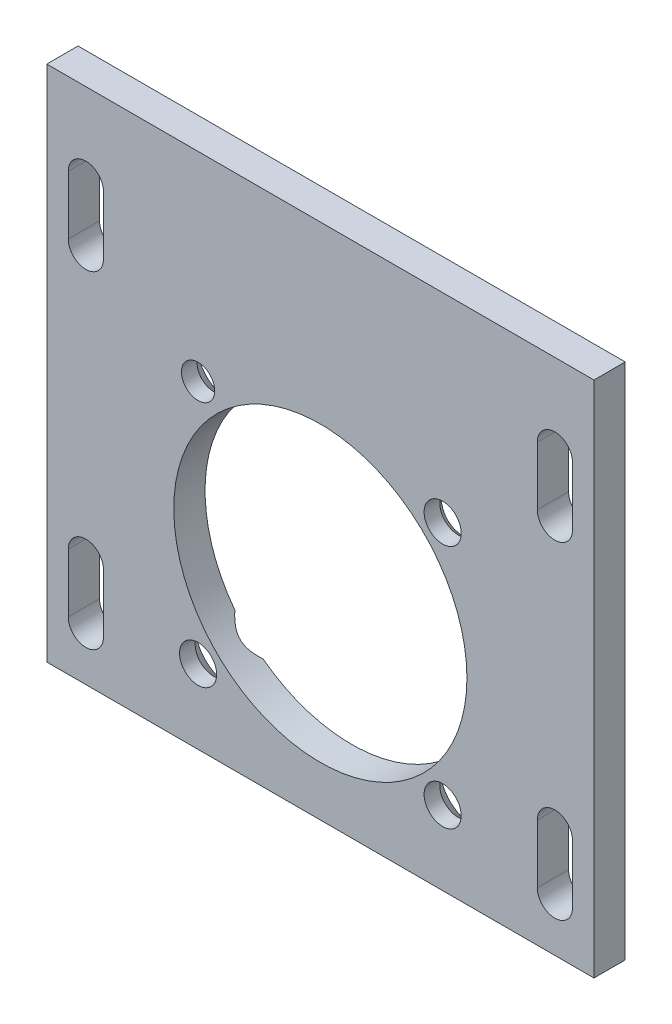
from build123d import *

# Parameters (mm, degrees)
SKETCH1_W                = 280
SKETCH1_H                = 280
SKETCH1_R                = 75
EXTRUDE1_DEPTH           = 8
SKETCH_2_2_R             = 8.5
SKETCH_2_2_R_2           = 9.5
EXTRUDE2_DEPTH           = 8
EXTRUDE4_START           = -8
SKETCH_2_2_2_R           = 8.5
EXTRUDE4_DEPTH           = 8
EXTRUDE4_DRAFT           = 45
SKETCH_2_2_2_R_2         = 9.5
EXTRUDE4_PROFILE_2_DEPTH = 8
EXTRUDE4_PROFILE_2_DRAFT = 45
EXTRUDE4_PROFILE_3_DEPTH = 8
EXTRUDE4_PROFILE_3_DRAFT = 45
EXTRUDE4_PROFILE_4_DEPTH = 8
EXTRUDE4_PROFILE_4_DRAFT = 45
SKETCH3_W                = 280
SKETCH3_H                = 15
EXTRUDE5_DEPTH           = 16


with BuildPart() as part:
    # Sketch1 → Extrude1 (new, symmetric)
    with BuildSketch(Plane.XY):
        with Locations((0, 24.5)):
            Rectangle(SKETCH1_W, SKETCH1_H)
        Circle(SKETCH1_R, mode=Mode.SUBTRACT)
        with BuildLine():
            Line((-129, 122.5), (-129, 92.5))
            ThreePointArc((-129, 92.5), (-120, 83.5), (-111, 92.5))
            Line((-111, 92.5), (-111, 122.5))
            ThreePointArc((-111, 122.5), (-120, 131.5), (-129, 122.5))
        make_face(mode=Mode.SUBTRACT)
        with BuildLine():
            Line((111, 122.5), (111, 92.5))
            ThreePointArc((111, 92.5), (120, 83.5), (129, 92.5))
            Line((129, 92.5), (129, 122.5))
            ThreePointArc((129, 122.5), (120, 131.5), (111, 122.5))
        make_face(mode=Mode.SUBTRACT)
        with BuildLine():
            Line((-129, -45), (-129, -75))
            ThreePointArc((-129, -75), (-120, -84), (-111, -75))
            Line((-111, -75), (-111, -45))
            ThreePointArc((-111, -45), (-120, -36), (-129, -45))
        make_face(mode=Mode.SUBTRACT)
        with BuildLine():
            Line((111, -45), (111, -75))
            ThreePointArc((111, -75), (120, -84), (129, -75))
            Line((129, -75), (129, -45))
            ThreePointArc((129, -45), (120, -36), (111, -45))
        make_face(mode=Mode.SUBTRACT)
    extrude(amount=EXTRUDE1_DEPTH, both=True)

    # Sketch 2_2 → Extrude2 (cut)
    with BuildSketch(Plane.XY.offset(8)):
        with Locations((-62.578950135, 62.578950135)):
            Circle(SKETCH_2_2_R)
        with Locations((62.578950135, 62.578950135)):
            Circle(SKETCH_2_2_R_2)
        with Locations((62.578950135, -62.578950135)):
            Circle(SKETCH_2_2_R_2)
        with Locations((-62.578950135, -62.578950135)):
            Circle(SKETCH_2_2_R_2)
    extrude(amount=-EXTRUDE2_DEPTH, mode=Mode.SUBTRACT)


with BuildPart() as extrude4_tool:
    # Sketch 2_2 2 → Extrude4 (with draft: the straight prism first)
    with BuildSketch(Plane.XY.offset(8).offset(EXTRUDE4_START)):
        with Locations((-62.578950135, 62.578950135)):
            Circle(SKETCH_2_2_2_R)
    extrude(amount=-EXTRUDE4_DEPTH)
    # Extrude4: the draft: its side faces are tilted about the plane it starts from
    extrude4_sides = [extrude4_tool.faces().sort_by_distance(p)[0] for p in [
        (-71.078950135, 62.578950135, -4),
    ]]
    draft(extrude4_sides, Plane.XY.offset(8).offset(EXTRUDE4_START), EXTRUDE4_DRAFT)


with BuildPart() as part_1:
    add(part.part)

    # Extrude4: cut by extrude4_tool
    add(extrude4_tool.part, mode=Mode.SUBTRACT)


with BuildPart() as extrude4_profile_2_tool:
    # Sketch 2_2 2 → Extrude4 profile 2 (with draft: the straight prism first)
    with BuildSketch(Plane.XY.offset(8).offset(EXTRUDE4_START)):
        with Locations((62.578950135, 62.578950135)):
            Circle(SKETCH_2_2_2_R_2)
    extrude(amount=-EXTRUDE4_PROFILE_2_DEPTH)
    # Extrude4 profile 2: the draft: its side faces are tilted about the plane it starts from
    extrude4_profile_2_sides = [extrude4_profile_2_tool.faces().sort_by_distance(p)[0] for p in [
        (53.078950135, 62.578950135, -4),
    ]]
    draft(extrude4_profile_2_sides, Plane.XY.offset(8).offset(EXTRUDE4_START), EXTRUDE4_PROFILE_2_DRAFT)


with BuildPart() as part_2:
    add(part_1.part)

    # Extrude4 profile 2: cut by extrude4_profile_2_tool
    add(extrude4_profile_2_tool.part, mode=Mode.SUBTRACT)


with BuildPart() as extrude4_profile_3_tool:
    # Sketch 2_2 2 → Extrude4 profile 3 (with draft: the straight prism first)
    with BuildSketch(Plane.XY.offset(8).offset(EXTRUDE4_START)):
        with Locations((62.578950135, -62.578950135)):
            Circle(SKETCH_2_2_2_R_2)
    extrude(amount=-EXTRUDE4_PROFILE_3_DEPTH)
    # Extrude4 profile 3: the draft: its side faces are tilted about the plane it starts from
    extrude4_profile_3_sides = [extrude4_profile_3_tool.faces().sort_by_distance(p)[0] for p in [
        (53.078950135, -62.578950135, -4),
    ]]
    draft(extrude4_profile_3_sides, Plane.XY.offset(8).offset(EXTRUDE4_START), EXTRUDE4_PROFILE_3_DRAFT)


with BuildPart() as part_3:
    add(part_2.part)

    # Extrude4 profile 3: cut by extrude4_profile_3_tool
    add(extrude4_profile_3_tool.part, mode=Mode.SUBTRACT)


with BuildPart() as extrude4_profile_4_tool:
    # Sketch 2_2 2 → Extrude4 profile 4 (with draft: the straight prism first)
    with BuildSketch(Plane.XY.offset(8).offset(EXTRUDE4_START)):
        with Locations((-62.578950135, -62.578950135)):
            Circle(SKETCH_2_2_2_R_2)
    extrude(amount=-EXTRUDE4_PROFILE_4_DEPTH)
    # Extrude4 profile 4: the draft: its side faces are tilted about the plane it starts from
    extrude4_profile_4_sides = [extrude4_profile_4_tool.faces().sort_by_distance(p)[0] for p in [
        (-72.078950135, -62.578950135, -4),
    ]]
    draft(extrude4_profile_4_sides, Plane.XY.offset(8).offset(EXTRUDE4_START), EXTRUDE4_PROFILE_4_DRAFT)


with BuildPart() as part_4:
    add(part_3.part)

    # Extrude4 profile 4: cut by extrude4_profile_4_tool
    add(extrude4_profile_4_tool.part, mode=Mode.SUBTRACT)

    # Sketch3 → Extrude5 (cut)
    with BuildSketch(Plane.XY.offset(8)):
        with Locations((0, -108)):
            Rectangle(SKETCH3_W, SKETCH3_H)
    extrude(amount=-EXTRUDE5_DEPTH, mode=Mode.SUBTRACT)


solid = part_4.part
